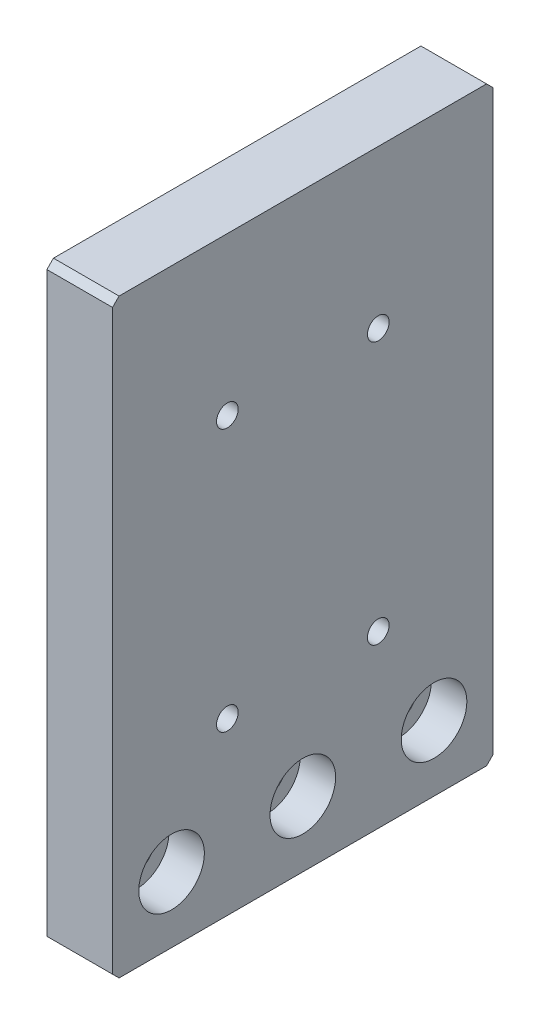
from build123d import *

# Parameters (mm, degrees)
SKETCH_1_W                   = 58
SKETCH_1_H                   = 90
EXTRUDE_1_DEPTH              = 10
HOLE_WIZARD_M4_1_D           = 3.3
HOLE_WIZARD_M5_1_D           = 5.5
HOLE_WIZARD_M5_1_CBORE_D     = 10
HOLE_WIZARD_M5_1_CBORE_DEPTH = 5.4
CHAMFER_1_SIZE               = 1


with BuildPart() as part:
    # 草图1 → 凸台-拉伸1 (new body)
    with BuildSketch(Plane(origin=(0, 0, 0), x_dir=(0, 0, -1), z_dir=(1, 0, 0))):
        Rectangle(SKETCH_1_W, SKETCH_1_H)
    extrude(amount=EXTRUDE_1_DEPTH)

    # M4 螺纹孔1 (through all)
    with Locations(Plane(origin=(10, 0, 0), x_dir=(0, 0, -1), z_dir=(1, 0, 0))):
        with Locations((-11.5, 21), (11.5, 21), (-11.5, -19), (11.5, -19)):
            Hole(HOLE_WIZARD_M4_1_D / 2)

    # M5 六角凹头螺钉的柱形沉头孔1 (through all)
    with Locations(Plane(origin=(10, 0, 0), x_dir=(0, 0, -1), z_dir=(1, 0, 0))):
        with Locations((-20, -35), (0, -35), (20, -35)):
            CounterBoreHole(HOLE_WIZARD_M5_1_D / 2, HOLE_WIZARD_M5_1_CBORE_D / 2, HOLE_WIZARD_M5_1_CBORE_DEPTH)

    # 倒角1
    chamfer_1_edges = [part.edges().sort_by_distance(p)[0] for p in [
        (5, -45, -29),
        (5, -45, 29),
        (5, 45, 29),
        (5, 45, -29),
    ]]
    chamfer(chamfer_1_edges, length=CHAMFER_1_SIZE)


solid = part.part
